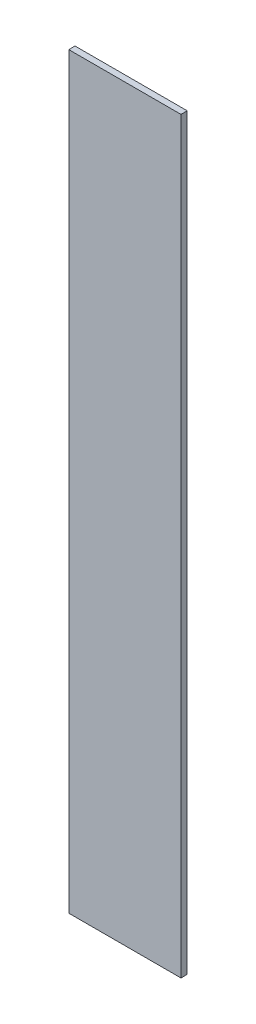
SolidWorks part; units mm, degrees
ref_plane "前视基准面" through (0, 0, 0) normal (0, 0, 1) x (1, 0, 0)
ref_plane "上视基准面" through (0, 0, 0) normal (0, 1, 0) x (1, 0, 0)
ref_plane "右视基准面" through (0, 0, 0) normal (1, 0, 0) x (0, 0, -1)
sketch "草图1" plane through (0, 0, 0) normal (0, 0, 1) x (1, 0, 0)
  line L0 (0, 0) -> (0, 600)
  line L1 (0, 600) -> (90, 600)
  line L2 (90, 600) -> (90, 0)
  line L3 (90, 0) -> (0, 0)
extrude "凸台-拉伸1" add sketch "草图1" along normal blind 3
sketch "草图2" plane through (0, 0, 0) normal (0, 0, -1) x (-1, 0, 0)
  line L8 (-90, 0) -> (0, 0)
  line L9 (0, 0) -> (0, 600)
  line L10 (0, 600) -> (-90, 600)
  line L11 (-90, 600) -> (-90, 0)
  line L12 (-90, 0) -> (0, 0)
  line L13 (0, 0) -> (0, 600)
  line L14 (0, 600) -> (-90, 600)
  line L15 (-90, 600) -> (-90, 0)
  dimension "D1" = 0
extrude "凸台-拉伸2" add sketch "草图2" along normal blind 2
